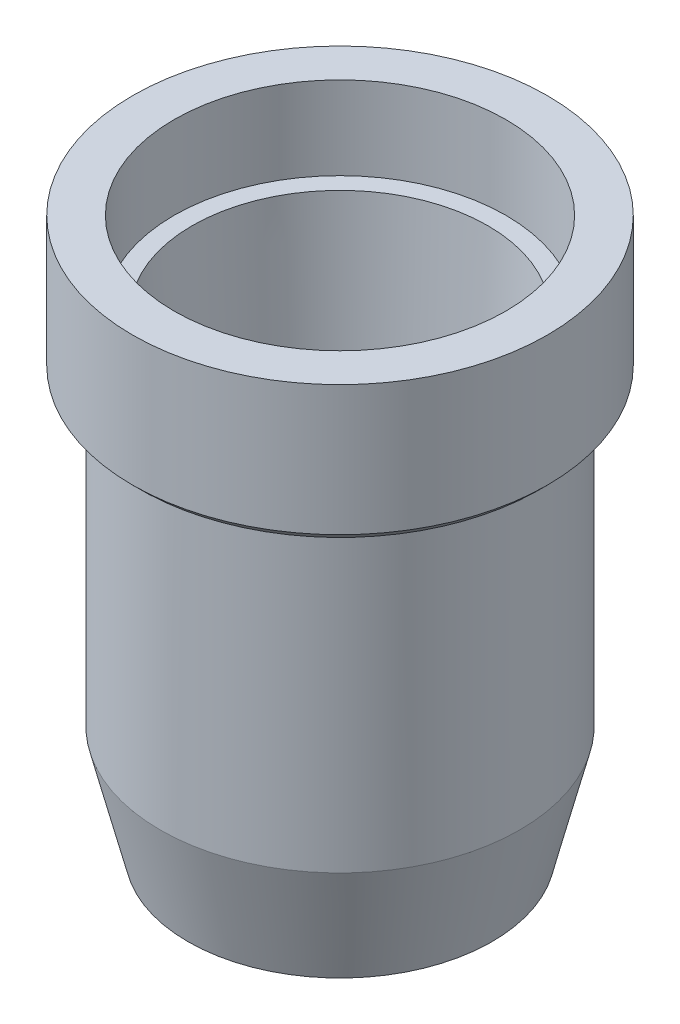
SolidWorks part; units mm, degrees
ref_plane "Front Plane" through (0, 0, 0) normal (0, 0, 1) x (1, 0, 0)
ref_plane "Top Plane" through (0, 0, 0) normal (0, 1, 0) x (1, 0, 0)
ref_plane "Right Plane" through (0, 0, 0) normal (1, 0, 0) x (0, 0, -1)
sketch "Sketch1" plane through (0, 0, 0) normal (0, 1, 0) x (1, 0, 0)
  circle A0 centre (0, 0) radius 7.5
  circle A1 centre (0, 0) radius 4.75
  dimension "D1" = 9.5
  dimension "D2" = 15
extrude "Boss-Extrude1" add sketch "Sketch1" along normal blind 20
sketch "Sketch2" plane through (0, 20, 0) normal (0, 1, 0) x (1, 0, 0)
  circle A0 centre (0, 0) radius 6
  dimension "D1" = 12
extrude "Cut-Extrude1" cut sketch "Sketch2" against normal blind 3
sketch "Sketch3" plane through (0, 0, 0) normal (0, -1, 0) x (1, 0, 0)
  circle A0 centre (0, 0) radius 6.5
  dimension "D1" = 13
extrude "Cut-Extrude2" cut sketch "Sketch3" against normal blind 15 flip side to cut
chamfer "Chamfer1" distance 0.6 distance2 10 1 edges at (0, 17, 4.75)
chamfer "Chamfer2" distance 0.3 angle 45 1 edges at (0, 15, -7.5)
chamfer "Chamfer3" distance 4 distance2 1 1 edges at (0, 0, -6.5)
